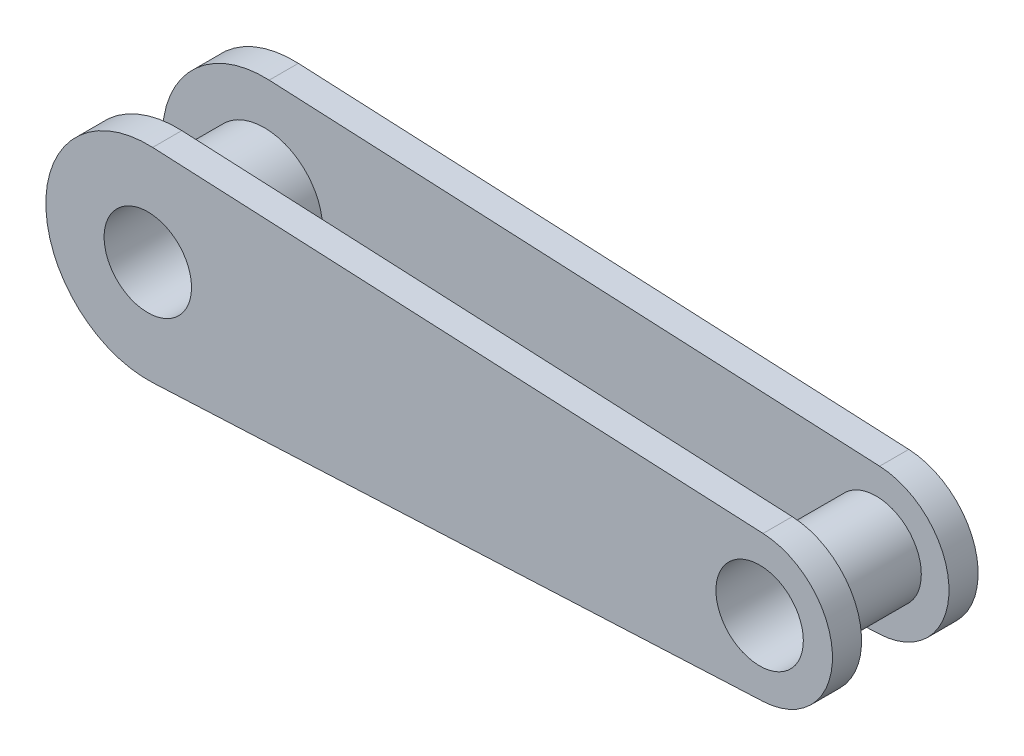
from build123d import *
from build123d.topology import SkipClean

# Parameters (mm, degrees)
BOSS_EXTRUDE1_DEPTH = 10
SKETCH3_R           = 20
SKETCH3_R_2         = 15
SKETCH3_R_3         = 15.5
BOSS_EXTRUDE2_DEPTH = 30
CUT_EXTRUDE1_START  = -106
SKETCH5_R           = 15
CUT_EXTRUDE1_DEPTH  = 106
BOSS_EXTRUDE3_START = 30
BOSS_EXTRUDE3_DEPTH = 10
SKETCH7_R           = 15
CUT_EXTRUDE2_DEPTH  = 110


with BuildPart() as part:
    # Sketch1 → Boss-Extrude1 (new body)
    with BuildSketch(Plane.XY):
        with BuildLine():
            Line((1.666666667, 34.960294939), (211.19047619, 24.971639242))
            ThreePointArc((211.19047619, 24.971639242), (235, 0), (211.19047619, -24.971639242))
            Line((211.19047619, -24.971639242), (1.666666667, -34.960294939))
            ThreePointArc((1.666666667, -34.960294939), (-35, 0), (1.666666667, 34.960294939))
        make_face()
    extrude(amount=BOSS_EXTRUDE1_DEPTH)

    # Sketch3 → Boss-Extrude2 (add)
    # profile 1 of 2: a face of its own
    with BuildSketch(Plane(origin=(0, 0, 0), x_dir=(-1, 0, 0), z_dir=(0, 0, -1))):
        with Locations(Location((0, 0, 0), (0, 0, 180))):
            Circle(SKETCH3_R)
        Circle(SKETCH3_R_2, mode=Mode.SUBTRACT)
    # profile 2 of 2: a face of its own
    with BuildSketch(Plane(origin=(0, 0, 0), x_dir=(-1, 0, 0), z_dir=(0, 0, -1))):
        with Locations(Location((-210, 0, 0), (0, 0, 180))):
            Circle(SKETCH3_R_3)
        with Locations((-210, 0)):
            Circle(SKETCH3_R_2, mode=Mode.SUBTRACT)
    extrude(amount=BOSS_EXTRUDE2_DEPTH)

    # Sketch5 → Cut-Extrude1 (cut)
    with SkipClean():  # the faces are left unmerged after this step: merging them gives an invalid solid
        with BuildSketch(Plane(origin=(0, 0, -30), x_dir=(-1, 0, 0), z_dir=(0, 0, -1)).offset(CUT_EXTRUDE1_START)):
            with Locations(Location((0, 0, 0), (0, 0, 180))):
                Circle(SKETCH5_R)
            with Locations(Location((-210, 0, 0), (0, 0, 180))):
                Circle(SKETCH5_R)
        extrude(amount=CUT_EXTRUDE1_DEPTH, mode=Mode.SUBTRACT)


with BuildPart() as body_2:
    # Sketch6 → Boss-Extrude3 (new body)
    with BuildSketch(Plane(origin=(0, 0, 0), x_dir=(-1, 0, 0), z_dir=(0, 0, -1)).offset(BOSS_EXTRUDE3_START)):
        with BuildLine():
            Line((-1.666666667, 34.960294939), (-211.19047619, 24.971639242))
            ThreePointArc((-211.19047619, 24.971639242), (-235, 0), (-211.19047619, -24.971639242))
            Line((-211.19047619, -24.971639242), (-1.666666667, -34.960294939))
            ThreePointArc((-1.666666667, -34.960294939), (35, 0), (-1.666666667, 34.960294939))
        make_face()
    extrude(amount=BOSS_EXTRUDE3_DEPTH)

    # Sketch7 → Cut-Extrude2 (cut)
    with BuildSketch(Plane.XY.offset(-30)):
        with Locations((210, 0)):
            Circle(SKETCH7_R)
        Circle(SKETCH7_R)
    extrude(amount=-CUT_EXTRUDE2_DEPTH, mode=Mode.SUBTRACT)


solid = Compound([part.part, body_2.part])
